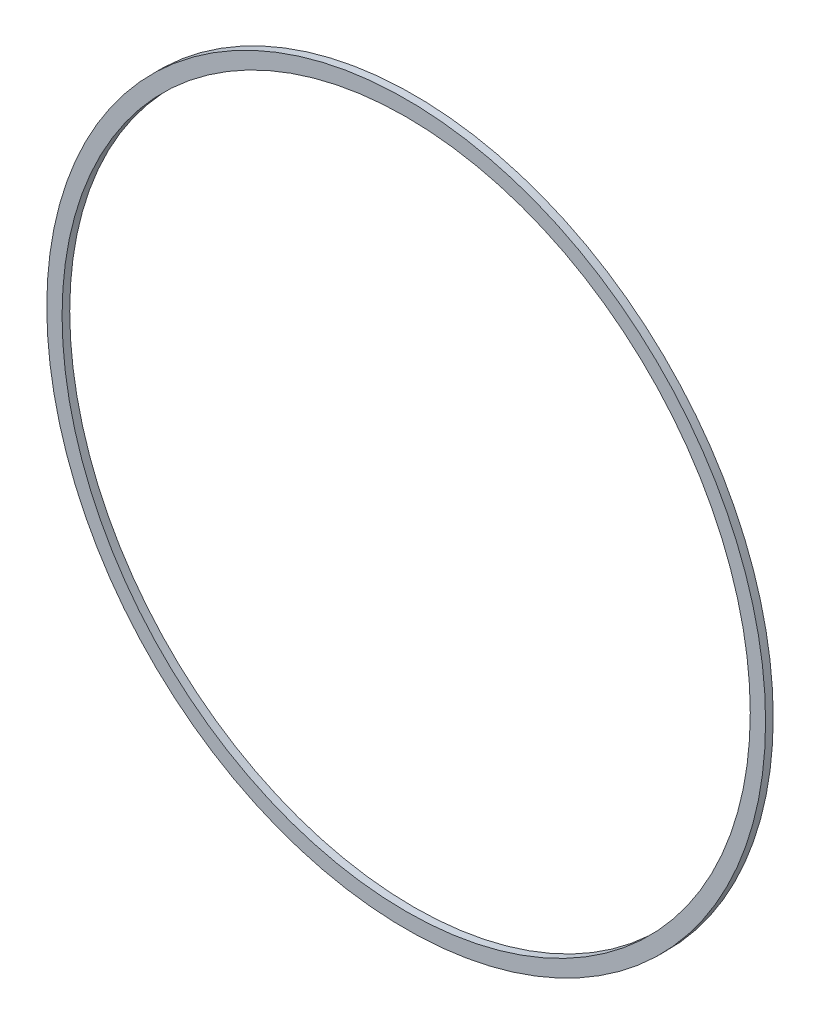
from build123d import *

# Parameters (mm, degrees)
SKETCH_1_R      = 94
SKETCH_1_R_2    = 90
EXTRUDE_1_DEPTH = 1


with BuildPart() as part:
    # 草图1 → 凸台-拉伸1 (new, symmetric)
    with BuildSketch(Plane.XY):
        Circle(SKETCH_1_R)
        Circle(SKETCH_1_R_2, mode=Mode.SUBTRACT)
    extrude(amount=EXTRUDE_1_DEPTH, both=True)


solid = part.part
